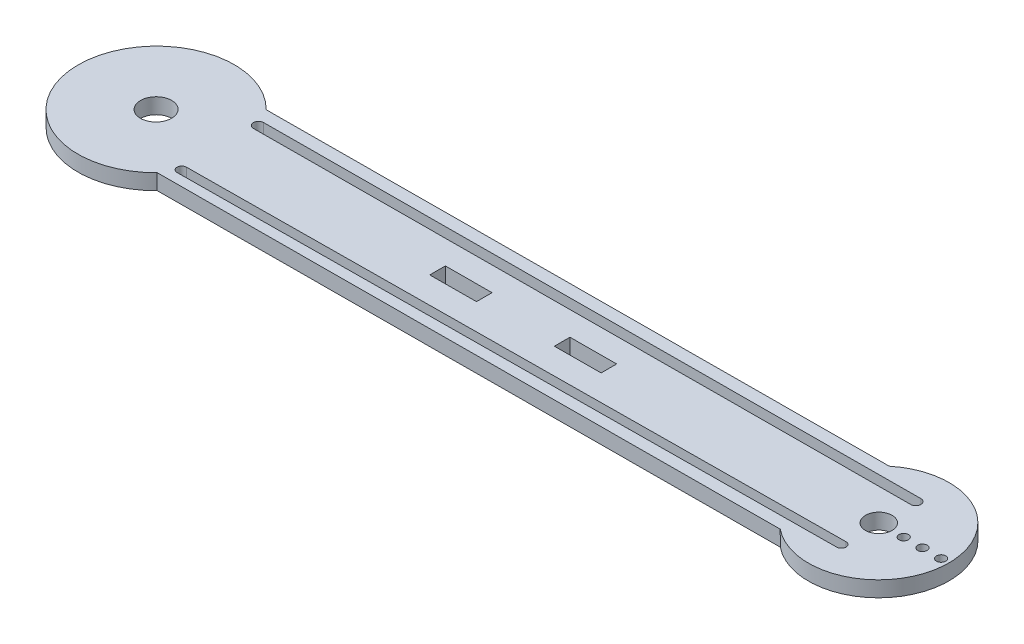
SolidWorks part; units mm, degrees
ref_plane "前视基准面" through (0, 0, 0) normal (0, 0, 1) x (1, 0, 0)
ref_plane "上视基准面" through (0, 0, 0) normal (0, 1, 0) x (1, 0, 0)
ref_plane "右视基准面" through (0, 0, 0) normal (1, 0, 0) x (0, 0, -1)
sketch "草图1" plane through (-1.4576, 322.1766, 0) normal (0.0045, -1, 0) x (1, 0.0045, 0)
  line L0 (87.0773, 423.8137) -> (-112.9227, 423.8137)
  line L1 (87.0773, 388.8137) -> (-112.9227, 388.8137)
  line L2 (101.2194, 406.3137) -> (54.4848, 406.3137) construction
  circle A1 centre (101.2194, 406.3137) radius 4.25
  arc A2 (87.0773, 388.8137) -> (87.0773, 423.8137) centre (101.2194, 406.3137) ccw
  arc A3 (-112.9227, 423.8137) -> (-112.9227, 388.8137) centre (-130.7763, 406.3137) ccw
  circle A4 centre (-130.7763, 406.3137) radius 5
  dimension "D1" = 45
  dimension "D3" = 50
  dimension "D4" = 10
  dimension "D5" = 200
  dimension "D6" = 8.5
  dimension "D2" = 35
extrude "凸台-拉伸1" add sketch "草图1" along normal blind 5
sketch "草图2" plane through (-1.4576, 322.1766, 0) normal (-0.0045, 1, 0) x (1, 0.0045, 0)
  line L0 (101.2194, -406.3137) -> (-34.0036, -406.3137) construction
  circle A0 centre (101.2194, -406.3137) radius 4.25 construction
  circle A1 centre (101.2194, -406.3137) radius 4.25
  circle A2 centre (101.2194, -406.3137) radius 20 construction
  circle A3 centre (121.2194, -406.3137) radius 1.5
  circle A4 centre (115.2194, -406.3137) radius 1.5
  circle A5 centre (109.2194, -406.3137) radius 1.5
  circle A6 centre (-41.2142, -347.7912) radius 1.5
  circle A7 centre (-45.4569, -343.5486) radius 1.5
  circle A8 centre (-49.6995, -339.3059) radius 1.5
  circle A9 centre (-114.6905, -191.5516) radius 1.5
  circle A10 centre (-114.6905, -185.5516) radius 1.5
  circle A11 centre (-114.6905, -179.5516) radius 1.5
  circle A12 centre (-56.168, -29.118) radius 1.5
  circle A13 centre (-51.9254, -24.8753) radius 1.5
  circle A14 centre (-47.6827, -20.6327) radius 1.5
  circle A15 centre (100.0716, 44.3583) radius 1.5
  circle A16 centre (106.0716, 44.3583) radius 1.5
  circle A17 centre (112.0716, 44.3583) radius 1.5
  circle A18 centre (262.5052, -14.1642) radius 1.5
  circle A19 centre (266.7478, -18.4068) radius 1.5
  circle A20 centre (270.9905, -22.6494) radius 1.5
  circle A21 centre (335.9815, -170.4037) radius 1.5
  circle A22 centre (335.9815, -176.4037) radius 1.5
  circle A23 centre (335.9815, -182.4037) radius 1.5
  circle A24 centre (277.459, -332.8374) radius 1.5
  circle A25 centre (273.2164, -337.08) radius 1.5
  circle A26 centre (268.9737, -341.3227) radius 1.5
  dimension "D1" = 40
  dimension "D2" = 6
  dimension "D4" = 3
  dimension "D3" = 6
  dimension "D5" = 8
extrude "切除-拉伸1" cut sketch "草图2" against normal blind 10
sketch "草图3" plane through (-1.4576, 322.1766, 0) normal (-0.0045, 1, 0) x (1, 0.0045, 0)
  line L1 (-109.7579, -394.4478) -> (101.2194, -394.4478) construction
  line L2 (-109.7579, -392.8137) -> (101.2194, -392.8137)
  line L3 (-109.7579, -396.0819) -> (101.2194, -396.0819)
  line L4 (-112.9227, -388.8137) -> (87.0773, -388.8137) construction
  line L5 (-109.7579, -419.0929) -> (101.2139, -418.3137) construction
  line L6 (-109.7523, -420.5928) -> (101.2194, -419.8137)
  line L7 (-109.7634, -417.5929) -> (101.2084, -416.8137)
  arc A0 (-109.7579, -392.8137) -> (-109.7579, -396.0819) centre (-109.7579, -394.4478) ccw
  arc A1 (101.2194, -396.0819) -> (101.2194, -392.8137) centre (101.2194, -394.4478) ccw
  arc A2 (-109.7523, -420.5928) -> (-109.7634, -417.5929) centre (-109.7579, -419.0929) cw
  arc A3 (101.2084, -416.8137) -> (101.2194, -419.8137) centre (101.2139, -418.3137) cw
  point P6 (-4.2692, -394.4478)
  point P15 (-4.272, -418.7033)
  dimension "D1" = 4
extrude "切除-拉伸2" cut sketch "草图3" against normal blind 10
sketch "草图4" plane through (-1.4576, 322.1766, 0) normal (-0.0045, 1, 0) x (1, 0.0045, 0)
  line L0 (-12.9227, -388.8137) -> (-12.9227, -423.8137) construction
  line L1 (-40.4227, -408.8137) -> (-25.4227, -408.8137)
  line L2 (-40.4227, -408.8137) -> (-40.4227, -403.8137)
  line L3 (-40.4227, -403.8137) -> (-25.4227, -403.8137)
  line L4 (-25.4227, -408.8137) -> (-25.4227, -403.8137)
  line L5 (-0.4227, -408.8137) -> (14.5773, -408.8137)
  line L6 (-0.4227, -408.8137) -> (-0.4227, -403.8137)
  line L7 (-0.4227, -403.8137) -> (14.5773, -403.8137)
  line L8 (14.5773, -408.8137) -> (14.5773, -403.8137)
  line L9 (-112.9227, -388.8137) -> (87.0773, -388.8137) construction
  line L10 (87.0773, -423.8137) -> (-112.9227, -423.8137) construction
  line L11 (-12.9227, -406.3137) -> (30.439, -406.3137) construction
  dimension "D1" = 25
  dimension "D2" = 15
  dimension "D3" = 15
  dimension "D4" = 5
extrude "切除-拉伸3" cut sketch "草图4" against normal blind 10
